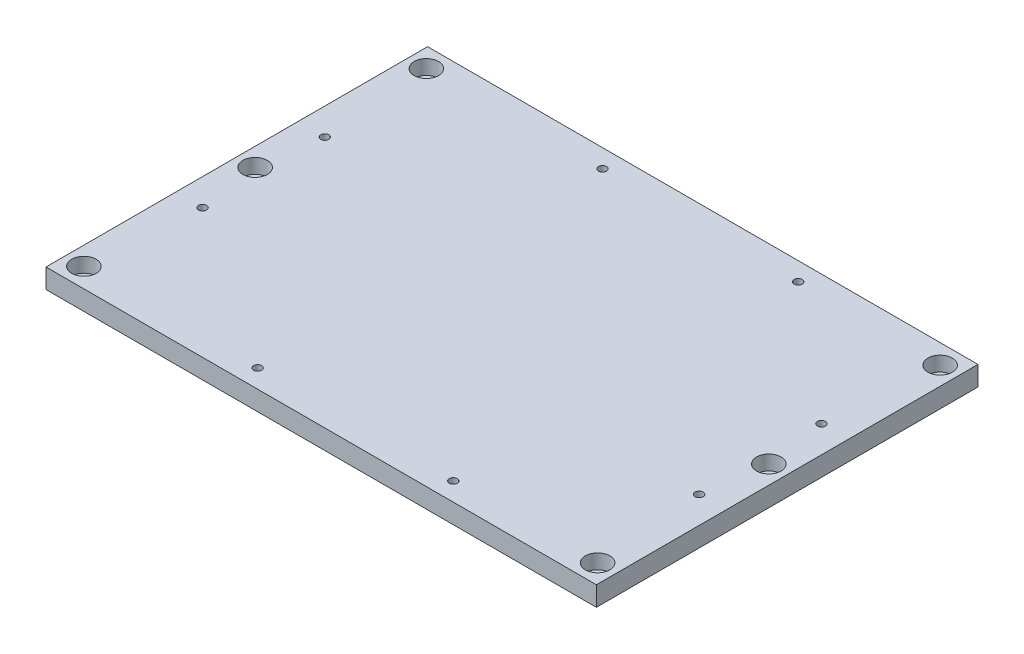
SolidWorks part; units mm, degrees
material "45#"
ref_plane "Front Plane" through (0, 0, 0) normal (0, 0, 1) x (1, 0, 0)
ref_plane "Top Plane" through (0, 0, 0) normal (0, 1, 0) x (1, 0, 0)
ref_plane "Right Plane" through (0, 0, 0) normal (1, 0, 0) x (0, 0, -1)
sketch "Sketch1" plane through (0, 0, 0) normal (0, 1, 0) x (1, 0, 0)
  line L0 (112.5, 78) -> (-112.5, -78) construction
  line L1 (-112.5, 78) -> (112.5, 78)
  line L2 (-112.5, 78) -> (-112.5, -78)
  line L3 (-112.5, -78) -> (112.5, -78)
  line L4 (112.5, 78) -> (112.5, -78)
  dimension "D1" = 225
  dimension "D2" = 156
extrude "Extrude1" add sketch "Sketch1" along normal mid plane 8
hole_wizard "M5 Socket Head Cap Screw Counterbore1" positions "3D Sketch1" profile "Sketch2" counterbore size "M5" standard "ISO" end condition through all
sketch3d "3D Sketch1"
  line L0 (112.5, 4, 0) -> (105, 4, 0) construction
  line L1 (112.5, 4, 78) -> (112.5, 4, -78) construction
  line L2 (105, 4, 0) -> (105, 4, -70) construction
  line L6 (105, 4, 70) -> (105, 4, 0) construction
  point P0 (105, 4, 70)
  point P2 (105, 4, 0)
  point P4 (105, 4, -70)
  dimension "D1" = 7.5
  dimension "D2" = 140
sketch "Sketch2" plane through (105, 4, 70) normal (1, 0, 0) x (0, 0, 1)
  line L0 (0, 0) -> (0, 8)
  line L1 (0, 8) -> (2.75, 8)
  line L3 (2.75, 8) -> (2.75, 6)
  line L4 (2.75, 6) -> (5, 6)
  line L5 (5, 6) -> (5, 0)
  line L7 (5, 0) -> (0, 0)
  line L11 (0, -6.35) -> (0, 107.95) construction
  dimension "貫穿孔直徑" = 5.5
  dimension "貫穿孔深度" = 8
  dimension "柱孔直徑" = 10
  dimension "柱孔深度" = 6
mirror "Mirror1" about plane through (0, 0, 0) normal (1, 0, 0) of "M5 Socket Head Cap Screw Counterbore1"
sketch "Sketch4" plane through (0, 4, 0) normal (0, 1, 0) x (1, 0, 0)
  line L0 (96.5, -25) -> (106.5, -25) construction
  line L2 (96.5, 25) -> (106.5, 25) construction
hole_wizard "M4 Tapped Hole1" positions "3D Sketch2" profile "Sketch5" tap size "M4" standard "ISO" end condition through all
sketch3d "3D Sketch2"
  line L0 (96.5, 4, 25) -> (106.5, 4, 25) construction
  line L1 (96.5, 4, -25) -> (106.5, 4, -25) construction
  point P0 (101.5, 4, 25)
  point P2 (101.5, 4, -25)
sketch "Sketch5" plane through (101.5, 4, 25) normal (1, 0, 0) x (0, 0, 1)
  line L0 (0, 0) -> (0, 8)
  line L1 (0, 8) -> (1.65, 8)
  line L2 (1.65, 8) -> (1.65, 0)
  line L5 (1.65, 0) -> (0, 0)
  line L11 (0, -6.35) -> (0, 107.95) construction
  dimension "貫穿螺孔鑽直徑" = 3.3
  dimension "貫穿螺孔鑽深度" = 8
cosmetic thread "Cosmetic Thread1" parameters "D2"=4
cosmetic thread "Cosmetic Thread2" parameters "D2"=4
sketch "Sketch6" plane through (0, 4, 0) normal (0, 1, 0) x (1, 0, 0)
  line L0 (46.5, -73) -> (46.5, -68) construction
  line L1 (-33.5, -73) -> (-33.5, -68) construction
hole_wizard "M4 Tapped Hole2" positions "3D Sketch3" profile "Sketch7" tap size "M4" standard "ISO" end condition through all
sketch3d "3D Sketch3"
  line L0 (-33.5, 4, 73) -> (-33.5, 4, 68) construction
  line L4 (46.5, 4, 73) -> (46.5, 4, 68) construction
  point P0 (-33.5, 4, 70.5)
  point P2 (46.5, 4, 70.5)
sketch "Sketch7" plane through (-33.5, 4, 70.5) normal (1, 0, 0) x (0, 0, 1)
  line L0 (0, 0) -> (0, 8)
  line L1 (0, 8) -> (1.65, 8)
  line L2 (1.65, 8) -> (1.65, 0)
  line L5 (1.65, 0) -> (0, 0)
  line L11 (0, -6.35) -> (0, 107.95) construction
  dimension "貫穿螺孔鑽直徑" = 3.3
  dimension "貫穿螺孔鑽深度" = 8
cosmetic thread "Cosmetic Thread3" parameters "D2"=4
cosmetic thread "Cosmetic Thread4" parameters "D2"=4
mirror "Mirror2" about plane through (0, 0, 0) normal (1, 0, 0) of "M4 Tapped Hole1"
mirror "Mirror3" about plane through (0, 0, 0) normal (0, 0, 1) of "M4 Tapped Hole2"
sketch "草图1" plane through (0, 4, 0) normal (0, 1, 0) x (1, 0, 0)
  circle A0 centre (0, 0) radius 38.9575
